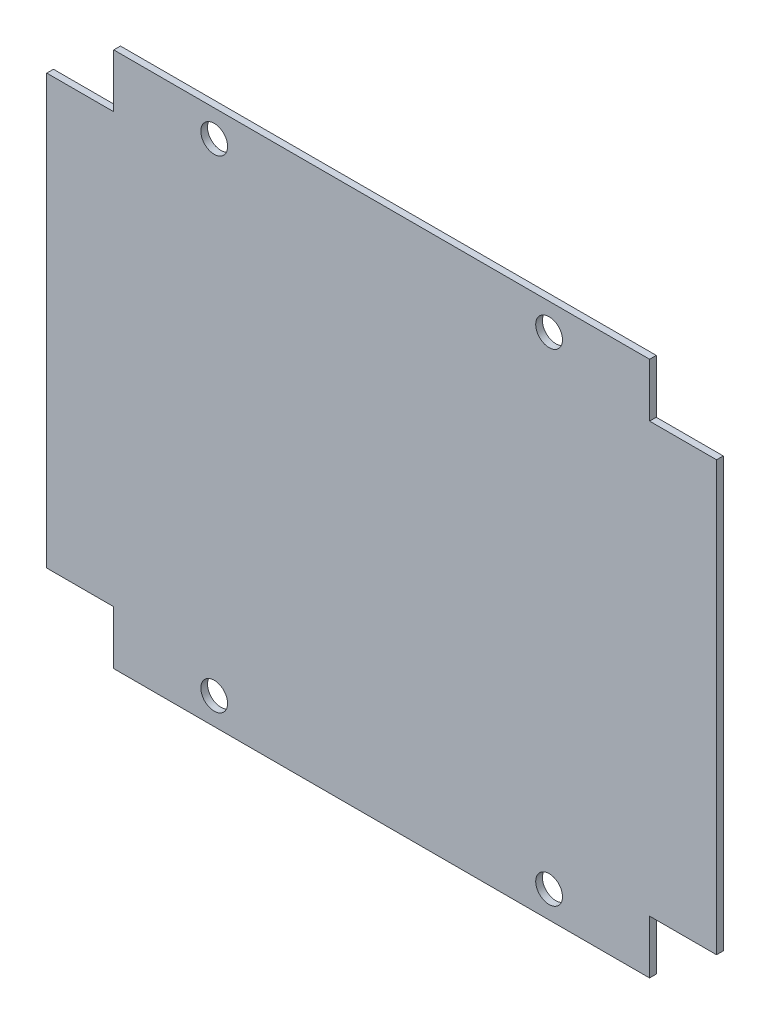
from build123d import *

# Parameters (mm, degrees)
SKETCH1_R           = 2
BOSS_EXTRUDE1_DEPTH = 1


with BuildPart() as part:
    # Sketch1 → Boss-Extrude1 (new body)
    with BuildSketch(Plane.XY):
        Polygon((-40, 40), (40, 40), (40, 32), (50, 32), (50, -32), (40, -32), (40, -40), (-40, -40), (-40, -32), (-50, -32), (-50, 32), (-40, 32), align=None)
        with Locations((-25, 36)):
            Circle(SKETCH1_R, mode=Mode.SUBTRACT)
        with Locations((-25, -36)):
            Circle(SKETCH1_R, mode=Mode.SUBTRACT)
        with Locations((25, 36)):
            Circle(SKETCH1_R, mode=Mode.SUBTRACT)
        with Locations((25, -36)):
            Circle(SKETCH1_R, mode=Mode.SUBTRACT)
    extrude(amount=BOSS_EXTRUDE1_DEPTH)


solid = part.part
